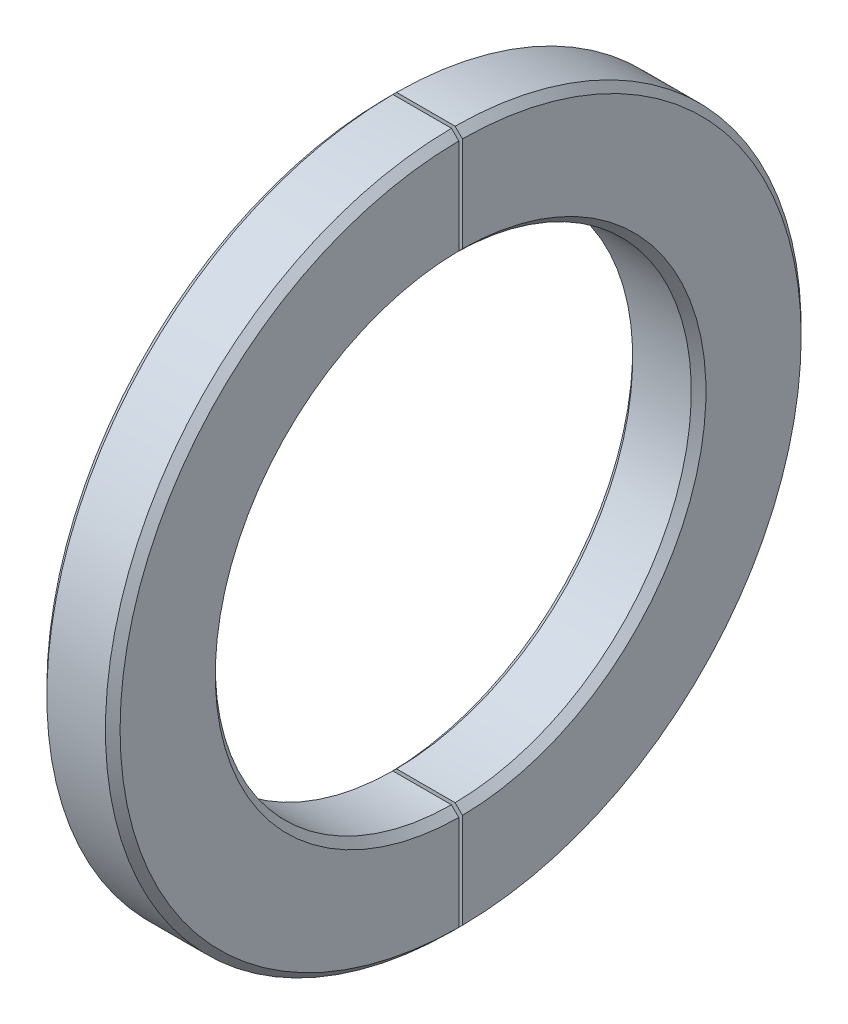
from build123d import *

# Parameters (mm, degrees)
SKETCH_1_R          = 47.5
SKETCH_1_R_2        = 32.5
EXTRUDE_1_DEPTH     = 10
CHAMFER_1_SIZE      = 1
SKETCH_2_W          = 0.5
SKETCH_2_H          = 159.347280508
CUT_EXTRUDE_1_DEPTH = 68.915388536


with BuildPart() as part:
    # 草图1 → 凸台-拉伸1 (new body)
    with BuildSketch(Plane(origin=(0, 0, 0), x_dir=(0, 0, -1), z_dir=(1, 0, 0))):
        Circle(SKETCH_1_R)
        Circle(SKETCH_1_R_2, mode=Mode.SUBTRACT)
    extrude(amount=EXTRUDE_1_DEPTH)

    # 倒角1
    chamfer_1_edges = [part.edges().sort_by_distance(p)[0] for p in [
        (0, 0, 47.5),
        (10, 0, 47.5),
        (0, 0, 32.5),
        (10, 0, 32.5),
    ]]
    chamfer(chamfer_1_edges, length=CHAMFER_1_SIZE)

    # 草图2 → 切除-拉伸1 (cut, through all)
    with BuildSketch(Plane.ZY):
        Rectangle(SKETCH_2_W, SKETCH_2_H)
    extrude(amount=-CUT_EXTRUDE_1_DEPTH, mode=Mode.SUBTRACT)


with BuildPart() as cut_extrude_1_piece_1:
    # of the separate pieces the step leaves, piece 1, a body of its own (cut_extrude_1_pieces)
    add(part.part.solids().sort_by_distance((1, -47.499342101, -0.25))[0])


with BuildPart() as cut_extrude_1_piece_2:
    # of the separate pieces the step leaves, piece 2, a body of its own (cut_extrude_1_pieces)
    add(part.part.solids().sort_by_distance((1, 47.499342101, 0.25))[0])


solid = Compound([cut_extrude_1_piece_1.part, cut_extrude_1_piece_2.part])
